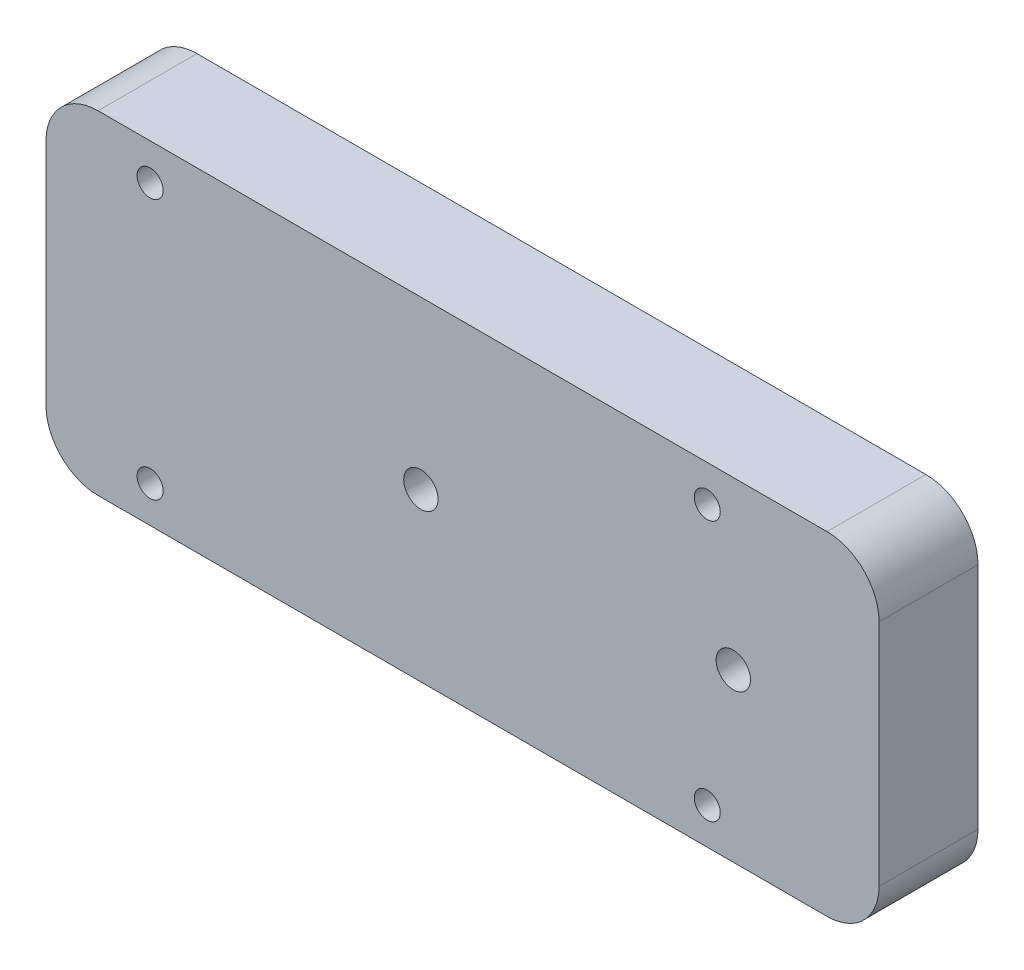
from build123d import *

# Parameters (mm, degrees)
SKETCH_1_W                = 160
SKETCH_1_H                = 64
EXTRUDE_1_DEPTH           = 19
FILLET_1_R                = 10
HOLE_WIZARD_M6_1_D        = 5
HOLE_WIZARD_2_D           = 6.6
HOLE_WIZARD_2_CSINK_D     = 12.8
HOLE_WIZARD_2_CSINK_ANGLE = 90


with BuildPart() as part:
    # 草图1 → 凸台-拉伸1 (new body)
    with BuildSketch(Plane.XY):
        Rectangle(SKETCH_1_W, SKETCH_1_H)
    extrude(amount=EXTRUDE_1_DEPTH)

    # 圆角1
    fillet_1_edges = [part.edges().sort_by_distance(p)[0] for p in [
        (80, -32, 9.5),
        (-80, -32, 9.5),
        (-80, 32, 9.5),
        (80, 32, 9.5),
    ]]
    fillet(fillet_1_edges, radius=FILLET_1_R)

    # M6 螺纹孔1 (through all)
    with Locations(Plane.XY.offset(19)):
        with Locations((-60, 25), (-60, -25), (47, 25), (47, -25)):
            Hole(HOLE_WIZARD_M6_1_D / 2)

    # 打孔尺寸(%根据)内六角花形半沉头螺钉的类型2 (through all)
    with Locations(Plane(origin=(0, 0, 0), x_dir=(-1, 0, 0), z_dir=(0, 0, -1))):
        with Locations((-52, 0), (8, 0)):
            CounterSinkHole(HOLE_WIZARD_2_D / 2, HOLE_WIZARD_2_CSINK_D / 2, counter_sink_angle=HOLE_WIZARD_2_CSINK_ANGLE)


solid = part.part
